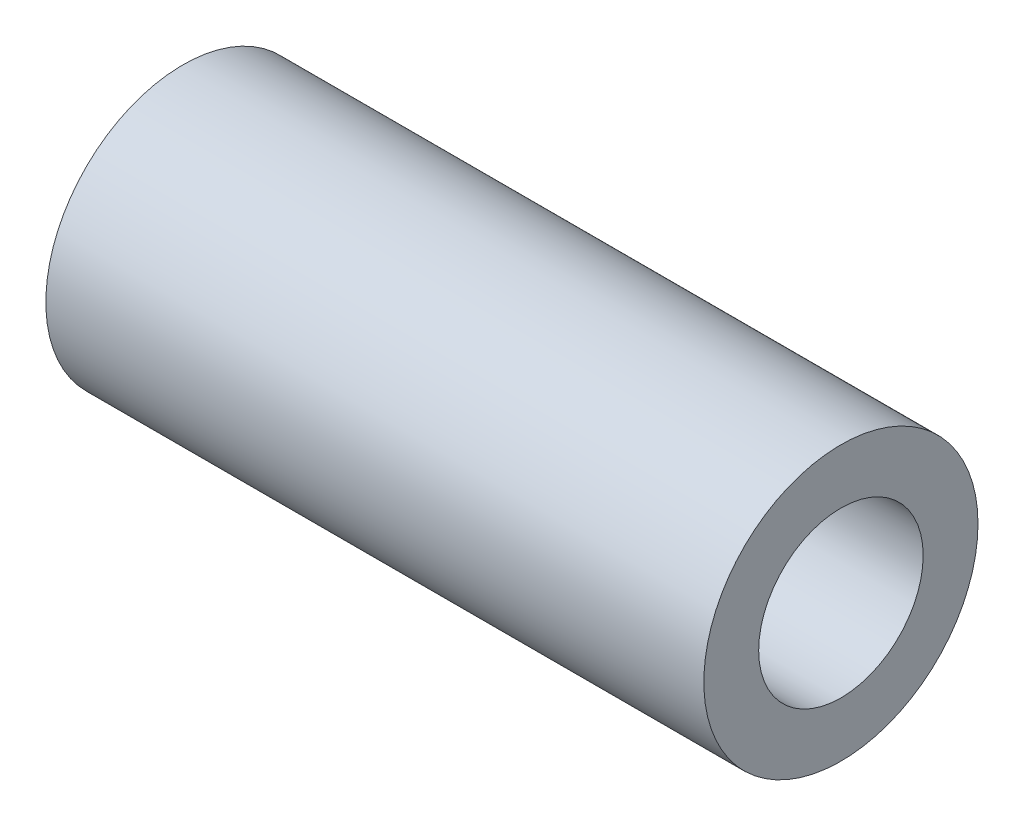
SolidWorks part; units mm, degrees
material "6061 合金"
ref_plane "前视基准面" through (0, 0, 0) normal (0, 0, 1) x (1, 0, 0)
ref_plane "上视基准面" through (0, 0, 0) normal (0, 1, 0) x (1, 0, 0)
ref_plane "右视基准面" through (0, 0, 0) normal (1, 0, 0) x (0, 0, -1)
other "Configuration Table"
sketch "草图1" plane through (0, 0, 0) normal (1, 0, 0) x (0, 0, -1)
  circle A0 centre (0, 0) radius 2.5
  circle A1 centre (0, 0) radius 1.5
  dimension "D1" = 5
  dimension "D2" = 3
extrude "凸台-拉伸1" add sketch "草图1" along normal blind 12
